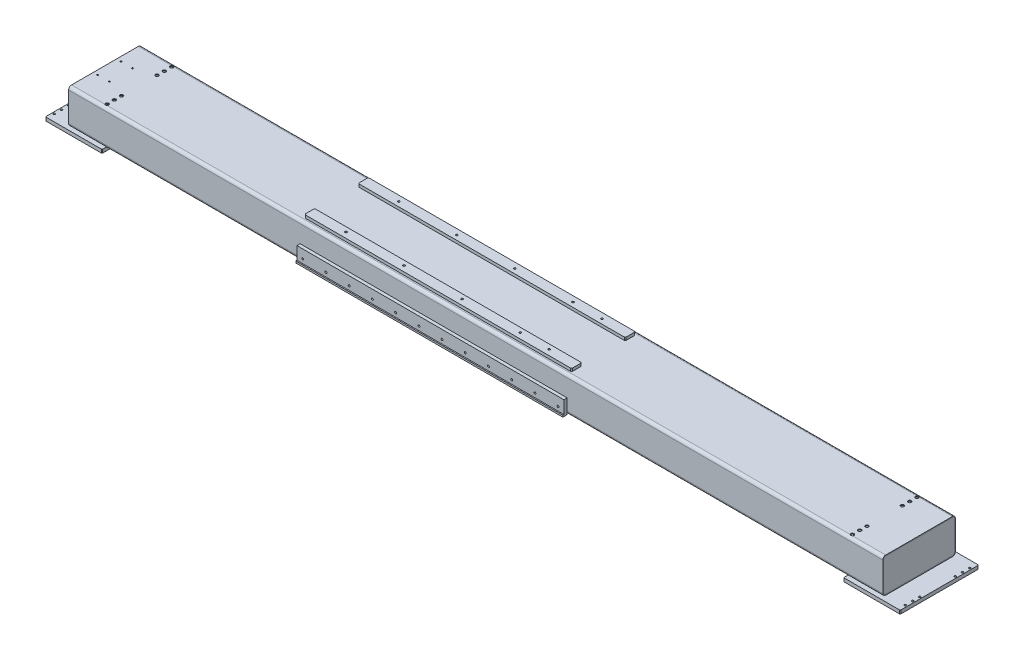
SolidWorks part; units mm, degrees
material "Q235A"
ref_plane "前基準面" through (0, 0, 0) normal (0, 0, 1) x (1, 0, 0)
ref_plane "上基準面" through (0, 0, 0) normal (0, 1, 0) x (1, 0, 0)
ref_plane "右基準面" through (0, 0, 0) normal (1, 0, 0) x (0, 0, -1)
sketch "草图1" plane through (0, 0, 0) normal (0, 1, 0) x (1, 0, 0)
  line L1 (-1402.5, 0) -> (1402.5, 0)
  point P0 (0, 0)
  dimension "D1" = 2805
other "矩型管 250 X 120 X 3.0(1)"
ref_plane "基准面1" through (-1402.5, 0, 0) normal (1, 0, 0) x (0, 1, 0)
sketch "Sketch11" plane through (-1402.5, 0, 0) normal (1, 0, 0) x (0, 1, 0)
  line L0 (-50, -122) -> (50, -122)
  line L1 (-57, -115) -> (-57, 115)
  line L2 (50, 122) -> (-50, 122)
  line L3 (57, 115) -> (57, -115)
  line L4 (-50, -125) -> (50, -125)
  line L5 (-60, -115) -> (-60, 115)
  line L6 (50, 125) -> (-50, 125)
  line L7 (60, 115) -> (60, -115)
  line L8 (-60, 0) -> (-57, 0) construction
  line L9 (-57, 0) -> (57, 0) construction
  line L10 (57, 0) -> (60, 0) construction
  line L11 (0, 125) -> (0, 122) construction
  line L12 (0, 122) -> (0, -122) construction
  line L13 (0, -122) -> (0, -125) construction
  arc A0 (60, 115) -> (50, 125) centre (50, 115) ccw
  arc A1 (50, -125) -> (60, -115) centre (50, -115) ccw
  arc A2 (-60, -115) -> (-50, -125) centre (-50, -115) ccw
  arc A3 (-50, 125) -> (-60, 115) centre (-50, 115) ccw
  arc A4 (-50, 122) -> (-57, 115) centre (-50, 115) ccw
  arc A5 (57, 115) -> (50, 122) centre (50, 115) ccw
  arc A6 (50, -122) -> (57, -115) centre (50, -115) ccw
  arc A7 (-57, -115) -> (-50, -122) centre (-50, -115) ccw
  point P6 (-60, 125)
  point P33 (-60, -125)
  point P34 (60, -125)
  point P36 (60, 125)
  point P37 (0, 0)
  dimension "D1" = 10
  dimension "Thickness" = 3
  dimension "V_leg" = 250
  dimension "H_leg" = 120
sketch "草图3" plane through (-1402.5, 0, 0) normal (-1, 0, 0) x (0, 0, 1)
  line L8 (-122, -50) -> (-122, 50) construction
  line L9 (122, 50) -> (122, -50) construction
  line L10 (-115, 57) -> (115, 57) construction
  line L11 (115, -57) -> (-115, -57) construction
  line L12 (-122, -50) -> (-122, 50)
  line L13 (122, 50) -> (122, -50)
  line L14 (-115, 57) -> (115, 57)
  line L15 (115, -57) -> (-115, -57)
  arc A8 (-122, -50) -> (-115, -57) centre (-115, -50) ccw construction
  arc A9 (-115, 57) -> (-122, 50) centre (-115, 50) ccw construction
  arc A10 (122, 50) -> (115, 57) centre (115, 50) ccw construction
  arc A11 (115, -57) -> (122, -50) centre (115, -50) ccw construction
  arc A12 (-122, -50) -> (-115, -57) centre (-115, -50) ccw
  arc A13 (-115, 57) -> (-122, 50) centre (-115, 50) ccw
  arc A14 (122, 50) -> (115, 57) centre (115, 50) ccw
  arc A15 (115, -57) -> (122, -50) centre (115, -50) ccw
extrude "凸台-拉伸1" add sketch "草图3" against normal blind 5 separate body
mirror "镜向1" about plane through (0, 0, 0) normal (0, 0, 1) of bodies 134
mirror "镜向2" about plane through (0, 0, 0) normal (1, 0, 0) of bodies 134 135
sketch "草图5" plane through (0, -60, -185) normal (0, -1, 0) x (1, 0, 0)
  line L1 (-1470.5, 320) -> (-1279.5, 320)
  line L2 (-1472.5, 318) -> (-1472.5, 52)
  line L3 (-1470.5, 50) -> (-1279.5, 50)
  line L4 (-1277.5, 318) -> (-1277.5, 52)
  line L5 (0, 732.875) -> (0, 185) construction
  line L6 (0, 185) -> (-1472.5, 185) construction
  line L7 (-1279.5, 320) -> (-1277.5, 318)
  line L8 (-1279.5, 50) -> (-1277.5, 52)
  line L9 (-1472.5, 52) -> (-1470.5, 50)
  line L10 (-1472.5, 318) -> (-1470.5, 320)
  line L11 (1472.5, 318) -> (1470.5, 320)
  line L12 (1472.5, 52) -> (1470.5, 50)
  line L13 (1279.5, 50) -> (1277.5, 52)
  line L14 (1279.5, 320) -> (1277.5, 318)
  line L15 (1277.5, 318) -> (1277.5, 52)
  line L16 (1470.5, 50) -> (1279.5, 50)
  line L17 (1472.5, 318) -> (1472.5, 52)
  line L18 (1470.5, 320) -> (1279.5, 320)
  line L19 (-1402.5, 70) -> (-1402.5, 300) construction
  point P0 (-1472.5, 320)
  point P1 (-1277.5, 50)
  point P2 (-1472.5, 50)
  point P3 (-1277.5, 320)
  point P28 (1277.5, 320)
  point P29 (1472.5, 50)
  point P30 (1277.5, 50)
  point P31 (1472.5, 320)
  dimension "D1" = 70
  dimension "D2" = 195
  dimension "D7" = 270
extrude "凸台-拉伸2" add sketch "草图5" along normal blind 12 separate body
hole_wizard "M8 间隙孔1" positions "草图7" profile "草图8" hole size "M8" standard "GB"
sketch "草图7" plane through (0, -40, 0) normal (0, 1, 0) x (1, 0, 0)
  line L0 (-1338.5, 56.5) -> (-1626.5, 56.5) construction
  line L1 (-1338.5, 241) -> (-1338.5, -128) construction
  line L2 (-1626.5, -128) -> (-1626.5, 241) construction
  line L4 (-1482.5, 56.5) -> (-1482.5, -186.4763) construction
  line L6 (0, 961.8145) -> (0, 0) construction
  point P0 (-1437.5, -18.5)
  point P2 (-1437.5, 56.5)
  point P16 (-1527.5, 56.5)
  point P17 (-1527.5, -18.5)
  point P18 (-1527.5, 131.5)
  point P21 (-1437.5, 131.5)
  point P27 (1527.5, -18.5)
  point P28 (1527.5, 56.5)
  point P29 (1437.5, 56.5)
  point P30 (1437.5, -18.5)
  point P31 (1437.5, 131.5)
  point P34 (1527.5, 131.5)
  dimension "D1" = 90
  dimension "D2" = 150
sketch "草图8" plane through (-1437.5, -40, 18.5) normal (1, 0, 0) x (0, 0, 1)
  line L0 (0, 0) -> (0, 12)
  line L1 (0, 12) -> (4.5, 12)
  line L2 (4.5, 12) -> (4.5, 0)
  line L5 (4.5, 0) -> (0, 0)
  line L11 (0, -6.35) -> (0, 107.95) construction
  dimension "通孔孔直径" = 9
  dimension "通孔孔深度" = 12
sketch "草图9" plane through (0, 60, 0) normal (0, 1, 0) x (1, 0, 0)
  line L0 (0, 0) -> (1745.0468, 0) construction
  line L1 (-605, 110) -> (315, 110)
  line L2 (-605, 110) -> (-605, 75)
  line L3 (-605, 75) -> (315, 75)
  line L4 (315, 110) -> (315, 75)
  line L5 (315, -110) -> (315, -75)
  line L6 (-605, -75) -> (315, -75)
  line L7 (-605, -110) -> (-605, -75)
  line L8 (-605, -110) -> (315, -110)
  line L9 (-1402.5, 115) -> (-1402.5, -115) construction
  dimension "D1" = 220
  dimension "D2" = 797.5
  dimension "D3" = 920
  dimension "D4" = 150
extrude "凸台-拉伸3" add sketch "草图9" along normal blind 10 separate body
hole_wizard "M8 螺纹孔1" positions "草图10" profile "草图11" tap size "M8" standard "GB"
sketch "草图10" plane through (0, 70, 0) normal (0, 1, 0) x (1, 0, 0)
  line L0 (0, 0) -> (1590.3364, 0) construction
  line L3 (-605, 110) -> (-605, 75) construction
  point P0 (-481, 91)
  point P9 (-481, -91)
  point P14 (-281, 91)
  point P15 (-281, -91)
  point P16 (-81, 91)
  point P17 (-81, -91)
  point P18 (119, 91)
  point P19 (119, -91)
  point P46 (319, -91) [skipped]
  point P47 (319, 91) [skipped]
  point P48 (219, -91)
  point P51 (219, 91)
  dimension "D1" = 5
  dimension "D2" = 182
  dimension "D3" = 200
  dimension "D4" = 124
  dimension "D5" = 100
sketch "草图11" plane through (-481, 70, -91) normal (1, 0, 0) x (0, 0, 1)
  line L0 (0, 0) -> (0, 21.7929)
  line L1 (0, 21.7929) -> (3.4, 19.75)
  line L2 (3.4, 19.75) -> (3.4, 0)
  line L5 (3.4, 0) -> (0, 0)
  line L10 (0, 21.7929) -> (-3.4, 19.75) construction
  line L11 (0, -6.35) -> (0, 107.95) construction
  dimension "螺纹孔钻头直径" = 6.8
  dimension "螺纹孔钻头深度" = 19.75
  dimension "导头角度" = 118
cosmetic thread "孔螺蚊线2" parameters "D1"=13, "D2"=8
cosmetic thread "孔螺蚊线12" parameters "D1"=13, "D2"=8
cosmetic thread "孔螺蚊线13" parameters "D1"=13, "D2"=8
cosmetic thread "孔螺蚊线14" parameters "D1"=13, "D2"=8
cosmetic thread "孔螺蚊线15" parameters "D1"=13, "D2"=8
cosmetic thread "孔螺蚊线26" parameters "D1"=13, "D2"=8
cosmetic thread "孔螺蚊线27" parameters "D1"=13, "D2"=8
cosmetic thread "孔螺蚊线28" parameters "D1"=13, "D2"=8
cosmetic thread "孔螺蚊线29" parameters "D1"=13, "D2"=8
cosmetic thread "孔螺蚊线30" parameters "D1"=13, "D2"=8
sketch "草图12" plane through (0, 65, 125) normal (0, 0, -1) x (1, 0, 0)
  line L0 (1402.5, 125) -> (-1402.5, 125) construction
  line L1 (-605, 125) -> (315, 125)
  line L2 (-605, 125) -> (-605, 75)
  line L3 (-605, 75) -> (315, 75)
  line L4 (315, 125) -> (315, 75)
  line L6 (-605, -5) -> (-605, 5) construction
  dimension "D1" = 0
  dimension "D2" = 920
  dimension "D3" = 50
extrude "凸台-拉伸4" add sketch "草图12" against normal blind 15 separate body
hole_wizard "M6 螺纹孔1" positions "草图17" profile "草图18" tap size "M6" standard "GB"
sketch "草图17" plane through (0, 0, -125) normal (0, 0, -1) x (-1, 0, 0)
  line L2 (145, 60) -> (145, 0) construction
  line L3 (-315, 60) -> (605, 60) construction
  line L4 (-1402.5, 60) -> (1402.5, 60) construction
  point P0 (-305, -15)
  point P5 (145, -15)
  point P6 (595, -15)
  dimension "D2" = 75
  dimension "D3" = 450
  dimension "D1" = 3
sketch "草图18" plane through (305, -15, -125) normal (1, 0, 0) x (0, 1, 0)
  line L0 (0, 0) -> (0, 16.5022)
  line L1 (0, 16.5022) -> (2.5, 15)
  line L2 (2.5, 15) -> (2.5, 0)
  line L5 (2.5, 0) -> (0, 0)
  line L10 (0, 16.5022) -> (-2.5, 15) construction
  line L11 (0, -6.35) -> (0, 107.95) construction
  dimension "螺纹孔钻头直径" = 5
  dimension "螺纹孔钻头深度" = 15
  dimension "导头角度" = 118
cosmetic thread "孔螺蚊线83" parameters "D1"=3, "D2"=6
cosmetic thread "孔螺蚊线84" parameters "D1"=3, "D2"=6
cosmetic thread "孔螺蚊线85" parameters "D1"=3, "D2"=6
hole_wizard "M6 螺纹孔2" positions "草图19" profile "草图20" tap size "M6" standard "GB"
sketch "草图19" plane through (-1470, 60, 0) normal (0, -1, 0) x (0, 0, -1)
  line L0 (0, 1470) -> (0, 61.3717) construction
  line L5 (115, 67.5) -> (-115, 67.5) construction
  point P0 (-40, 82.5)
  point P7 (40, 82.5)
  point P18 (-40, 122.5)
  point P20 (40, 122.5)
  dimension "D1" = 80
  dimension "D2" = 15
  dimension "D3" = 40
sketch "草图20" plane through (-1387.5, 60, 40) normal (1, 0, 0) x (0, 0, 1)
  line L0 (0, 0) -> (0, 16.5022)
  line L1 (0, 16.5022) -> (2.5, 15)
  line L2 (2.5, 15) -> (2.5, 0)
  line L5 (2.5, 0) -> (0, 0)
  line L10 (0, 16.5022) -> (-2.5, 15) construction
  line L11 (0, -6.35) -> (0, 107.95) construction
  dimension "螺纹孔钻头直径" = 5
  dimension "螺纹孔钻头深度" = 15
  dimension "导头角度" = 118
cosmetic thread "孔螺蚊线86" parameters "D1"=3, "D2"=6
cosmetic thread "孔螺蚊线87" parameters "D1"=3, "D2"=6
cosmetic thread "孔螺蚊线88" parameters "D1"=3, "D2"=6
cosmetic thread "孔螺蚊线89" parameters "D1"=3, "D2"=6
chamfer "倒角1" distance 3 angle 45 4 edges at (-605, 65, -75) (-605, 65, -110) (315, 65, -75) (315, 65, -110)
chamfer "倒角2" distance 3 angle 45 4 edges at (315, 65, 110) (315, 65, 75) (-605, 65, 75) (-605, 65, 110)
hole_wizard "M6 间隙孔1" positions "草图21" profile "草图22" hole size "M6" standard "GB"
sketch "草图21" plane through (0, -60, 0) normal (0, 1, 0) x (1, 0, 0)
  line L0 (-1472.5, 0) -> (-1277.5, 0) construction
  line L1 (-1472.5, -133) -> (-1472.5, 133) construction
  line L2 (-1277.5, 133) -> (-1277.5, -133) construction
  line L4 (-1375, 0) -> (-1375, 310.334) construction
  line L6 (0, 0) -> (0, 516.7396) construction
  point P0 (-1466, 61)
  point P6 (-1284, 61)
  point P8 (-1284, -61)
  point P10 (-1466, -61)
  point P49 (-1466, 0) [skipped]
  point P50 (-1284, 0) [skipped]
  point P51 (-1466, -86)
  point P53 (-1466, -111)
  point P56 (-1284, -111)
  point P57 (-1284, -86)
  point P58 (-1284, 86)
  point P59 (-1284, 111)
  point P60 (-1466, 111)
  point P61 (-1466, 86)
  point P62 (1466, 86)
  point P63 (1466, 111)
  point P64 (1284, 111)
  point P65 (1284, 86)
  point P66 (1284, 61)
  point P67 (1466, 61)
  point P68 (1284, -86)
  point P69 (1284, -111)
  point P70 (1466, -111)
  point P71 (1466, -86)
  point P72 (1466, -61)
  point P73 (1284, -61)
sketch "草图22" plane through (-1466, -60, -61) normal (1, 0, 0) x (0, 0, 1)
  line L0 (0, 0) -> (0, 12)
  line L1 (0, 12) -> (3.3, 12)
  line L2 (3.3, 12) -> (3.3, 0)
  line L5 (3.3, 0) -> (0, 0)
  line L11 (0, -6.35) -> (0, 107.95) construction
  dimension "通孔孔直径" = 6.6
  dimension "通孔孔深度" = 12
hole_wizard "打孔尺寸(%根据)内六角圆柱头螺钉的类型1" positions "草图24" profile "草图25" counterbore size "M6" standard "GB" end condition through all
sketch "草图24" plane through (0, 60, 0) normal (0, 1, 0) x (1, 0, 0)
  line L0 (0, 0) -> (0, -305.2074) construction
  point P18 (-1284, -61)
  point P24 (-1284, 61)
  point P33 (-1284, -86)
  point P36 (-1284, -111)
  point P39 (-1284, 86)
  point P42 (-1284, 111)
  point P46 (1284, 111)
  point P47 (1284, 86)
  point P48 (1284, -111)
  point P49 (1284, -86)
  point P50 (1284, 61)
  point P51 (1284, -61)
sketch "草图25" plane through (1284, 60, 61) normal (1, 0, 0) x (0, 0, 1)
  line L0 (0, 0) -> (0, 132)
  line L1 (0, 132) -> (3.3, 132)
  line L3 (3.3, 132) -> (3.3, 6.8)
  line L4 (3.3, 6.8) -> (5.5, 6.8)
  line L5 (5.5, 6.8) -> (5.5, 0)
  line L7 (5.5, 0) -> (0, 0)
  line L11 (0, -6.35) -> (0, 107.95) construction
  dimension "通孔孔直径" = 6.6
  dimension "通孔孔深度" = 132
  dimension "柱形沉头孔直径" = 11
  dimension "柱形沉头孔深度" = 6.8
ref_plane "基准面2" through (1375, 0, 0) normal (1, 0, 0) x (0, 0, -1)
mirror "镜向3" [suppressed] about plane through (0, 0, 0) normal (1, 0, 0)
sketch "草图26" plane through (0, 0, 140) normal (0, 0, 1) x (1, 0, 0)
  line L0 (315, -10) -> (315, -60) construction
  line L1 (-605, -10) -> (315, -10)
  line L2 (-605, -10) -> (-605, -54)
  line L3 (-605, -54) -> (315, -54)
  line L4 (315, -10) -> (315, -54)
  line L5 (315, -60) -> (-605, -60) construction
  dimension "D1" = 6
extrude "切除-拉伸1" cut sketch "草图26" against normal blind 4
hole_wizard "M8 螺纹孔2" positions "草图13" profile "草图14" tap size "M8" standard "GB"
sketch "草图13" plane through (0, 0, 136) normal (0, 0, 1) x (-1, 0, 0)
  line L3 (145, 60) -> (145, 10) construction
  line L4 (-315, 60) -> (605, 60) construction
  line L5 (605, 10) -> (-315, 10) construction
  line L6 (605, 54) -> (-315, 54) construction
  point P7 (585, 40)
  point P14 (505, 40)
  point P15 (425, 40)
  point P16 (345, 40)
  point P17 (265, 40)
  point P18 (185, 40)
  point P19 (105, 40)
  point P20 (25, 40)
  point P21 (-55, 40)
  point P22 (-135, 40)
  point P23 (-215, 40)
  point P50 (-295, 40)
  dimension "D1" = 12
  dimension "D2" = 14
  dimension "D3" = 80
sketch "草图14" plane through (-585, -40, 136) normal (1, 0, 0) x (0, -1, 0)
  line L0 (0, 0) -> (0, 21.7929)
  line L1 (0, 21.7929) -> (3.4, 19.75)
  line L2 (3.4, 19.75) -> (3.4, 0)
  line L5 (3.4, 0) -> (0, 0)
  line L10 (0, 21.7929) -> (-3.4, 19.75) construction
  line L11 (0, -6.35) -> (0, 107.95) construction
  dimension "螺纹孔钻头直径" = 6.8
  dimension "螺纹孔钻头深度" = 19.75
  dimension "导头角度" = 118
cosmetic thread "孔螺蚊线94" parameters "D1"=13, "D2"=8
cosmetic thread "孔螺蚊线95" parameters "D1"=13, "D2"=8
cosmetic thread "孔螺蚊线96" parameters "D1"=13, "D2"=8
cosmetic thread "孔螺蚊线97" parameters "D1"=13, "D2"=8
cosmetic thread "孔螺蚊线98" parameters "D1"=13, "D2"=8
cosmetic thread "孔螺蚊线99" parameters "D1"=13, "D2"=8
cosmetic thread "孔螺蚊线100" parameters "D1"=13, "D2"=8
cosmetic thread "孔螺蚊线101" parameters "D1"=13, "D2"=8
cosmetic thread "孔螺蚊线102" parameters "D1"=13, "D2"=8
cosmetic thread "孔螺蚊线103" parameters "D1"=13, "D2"=8
cosmetic thread "孔螺蚊线104" parameters "D1"=13, "D2"=8
cosmetic thread "孔螺蚊线105" parameters "D1"=13, "D2"=8
equation "\"D6@草图21\"=\"D5@草图21\""
